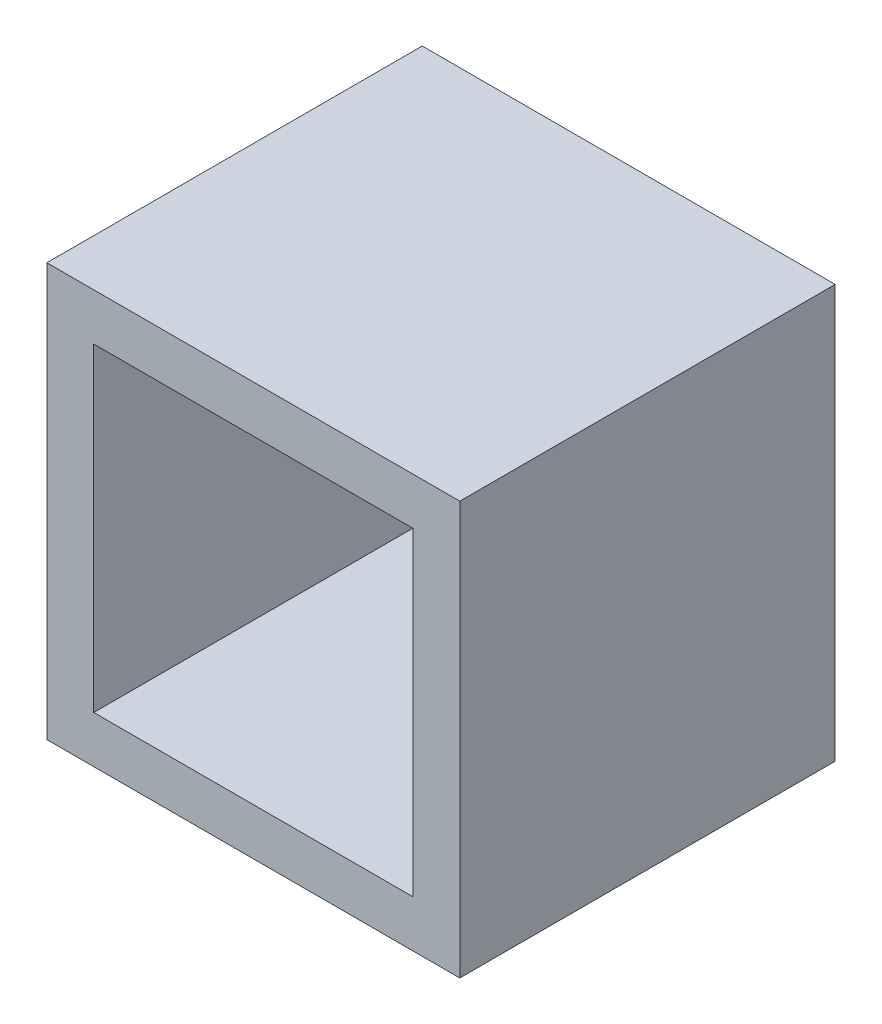
SolidWorks part; units mm, degrees
ref_plane "前视基准面" through (0, 0, 0) normal (0, 0, 1) x (1, 0, 0)
ref_plane "上视基准面" through (0, 0, 0) normal (0, 1, 0) x (1, 0, 0)
ref_plane "右视基准面" through (0, 0, 0) normal (1, 0, 0) x (0, 0, -1)
other "Configuration Table"
sketch "草图1" plane through (0, 0, 0) normal (0, 0, 1) x (1, 0, 0)
  line L0 (-33, -33) -> (33, -33)
  line L1 (33, -33) -> (33, 33)
  line L2 (33, 33) -> (-33, 33)
  line L3 (-33, 33) -> (-33, -33)
  line L4 (-25.5, -25.5) -> (25.5, -25.5)
  line L5 (25.5, -25.5) -> (25.5, 25.5)
  line L6 (25.5, 25.5) -> (-25.5, 25.5)
  line L7 (-25.5, 25.5) -> (-25.5, -25.5)
  point P0 (0, 0)
  dimension "D1" = 7.5
  dimension "D2" = 33
  dimension "D3" = 58.5
  dimension "D4" = 66
  dimension "D5" = 7.5
  dimension "D6" = 33
  dimension "D7" = 58.5
  dimension "D8" = 66
extrude "凸台-拉伸1" add sketch "草图1" against normal mid plane 60
